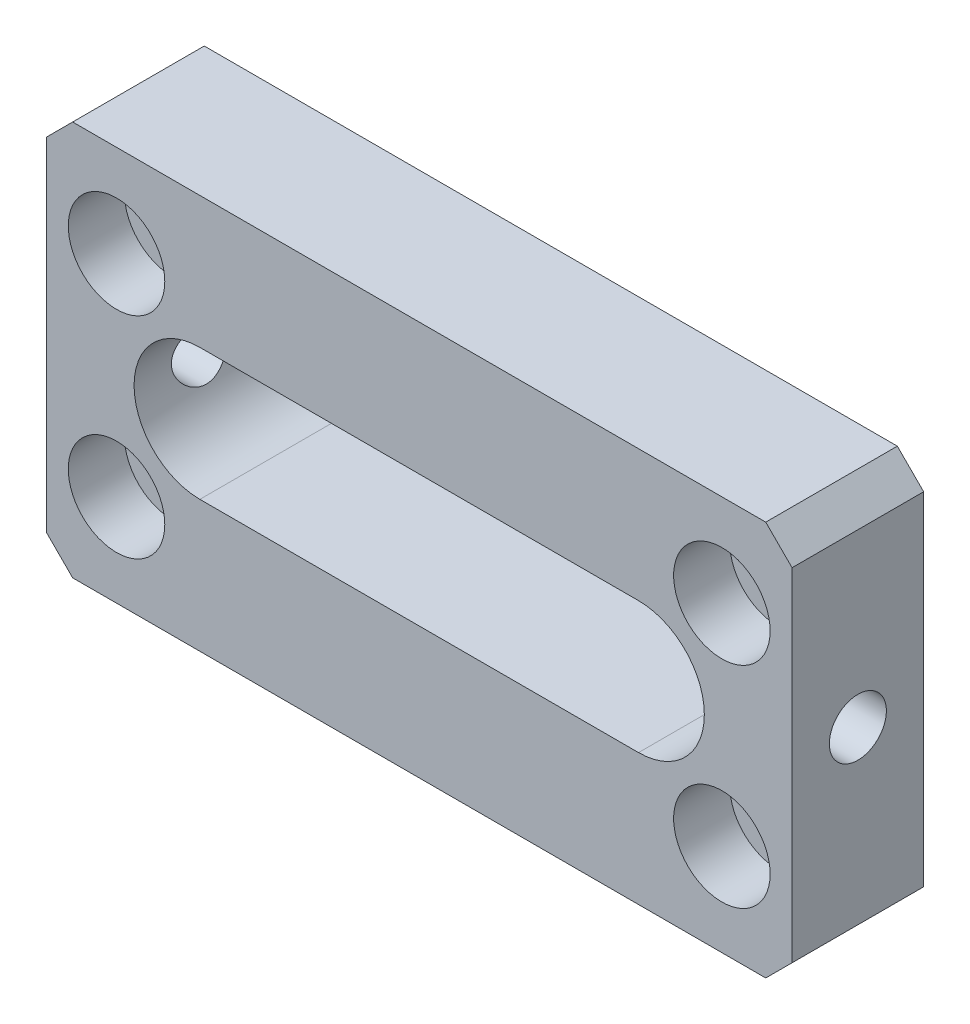
from build123d import *

# Parameters (mm, degrees)
SKETCH_1_W                   = 85
SKETCH_1_H                   = 45
EXTRUDE_1_DEPTH              = 15
HOLE_WIZARD_M6_1_D           = 6.6
HOLE_WIZARD_M6_1_CBORE_D     = 11
HOLE_WIZARD_M6_1_CBORE_DEPTH = 6.4
SKETCH_4_R                   = 3.25
CUT_EXTRUDE_1_DEPTH          = 162
CHAMFER_1_SIZE               = 3


with BuildPart() as part:
    # 草图1 → 凸台-拉伸1 (new body)
    with BuildSketch(Plane.XY):
        Rectangle(SKETCH_1_W, SKETCH_1_H)
        with BuildLine():
            Line((-25, 7.5), (25, 7.5))
            ThreePointArc((25, 7.5), (32.5, 0), (25, -7.5))
            Line((25, -7.5), (-25, -7.5))
            ThreePointArc((-25, -7.5), (-32.5, 0), (-25, 7.5))
        make_face(mode=Mode.SUBTRACT)
    extrude(amount=EXTRUDE_1_DEPTH)

    # M6 六角凹头螺钉的柱形沉头孔1 (through all)
    with Locations(Plane.XY.offset(15)):
        with Locations((-34.5, 12), (-34.5, -12), (34.5, -12), (34.5, 12)):
            CounterBoreHole(HOLE_WIZARD_M6_1_D / 2, HOLE_WIZARD_M6_1_CBORE_D / 2, HOLE_WIZARD_M6_1_CBORE_DEPTH)

    # 草图4 → 切除-拉伸1 (cut)
    with BuildSketch(Plane.ZY.offset(42.5)):
        with Locations((7.5, 0)):
            Circle(SKETCH_4_R)
    extrude(amount=-CUT_EXTRUDE_1_DEPTH, mode=Mode.SUBTRACT)

    # 倒角1
    chamfer_1_edges = [part.edges().sort_by_distance(p)[0] for p in [
        (42.5, -22.5, 7.5),
        (-42.5, -22.5, 7.5),
        (-42.5, 22.5, 7.5),
        (42.5, 22.5, 7.5),
    ]]
    chamfer(chamfer_1_edges, length=CHAMFER_1_SIZE)


solid = part.part
